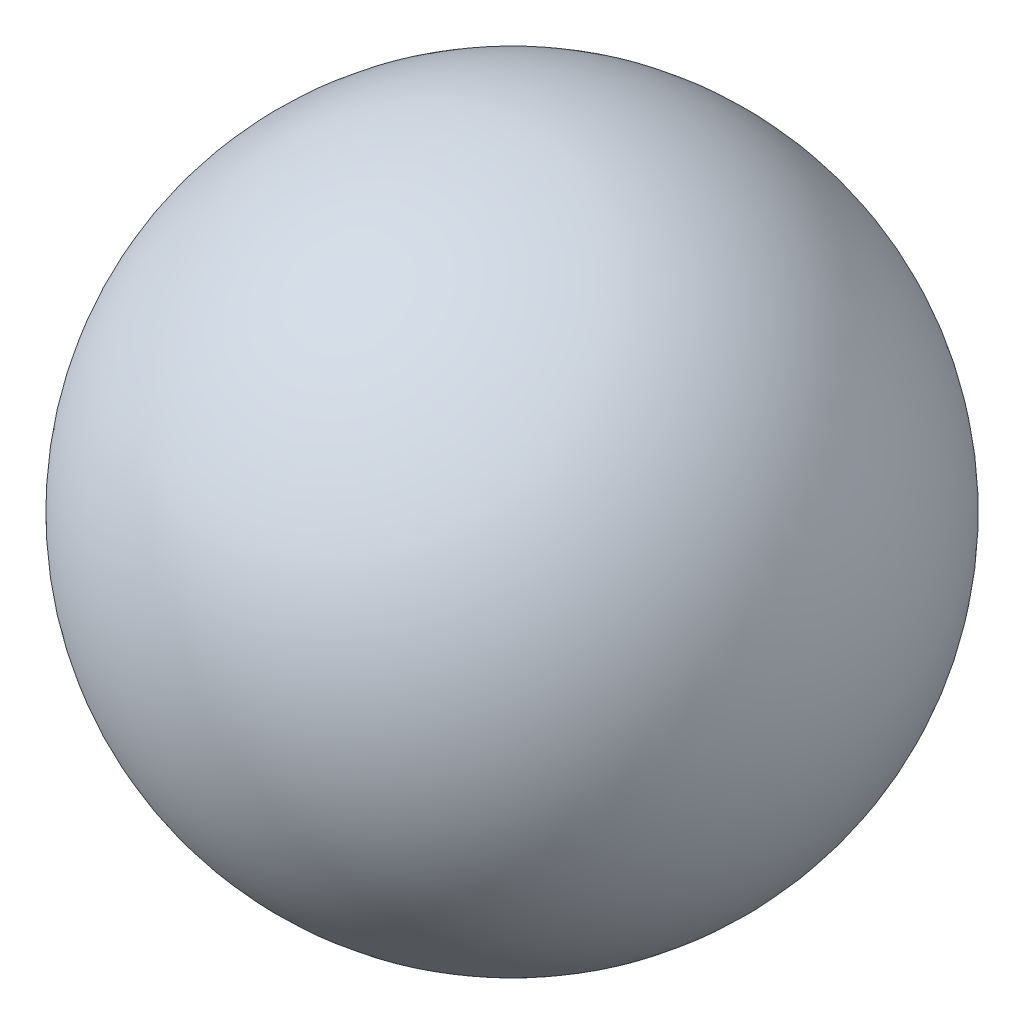
from build123d import *


with BuildPart() as part:
    # Sketch1 → Revolve1 (revolve)
    with BuildSketch(Plane.XY):
        with BuildLine():
            Line((0, 1.65), (0, -1.65))
            ThreePointArc((0, -1.65), (1.65, 0), (0, 1.65))
        make_face()
    revolve(axis=Axis((0, 1.65, 0), (0, -1, 0)))


solid = part.part
